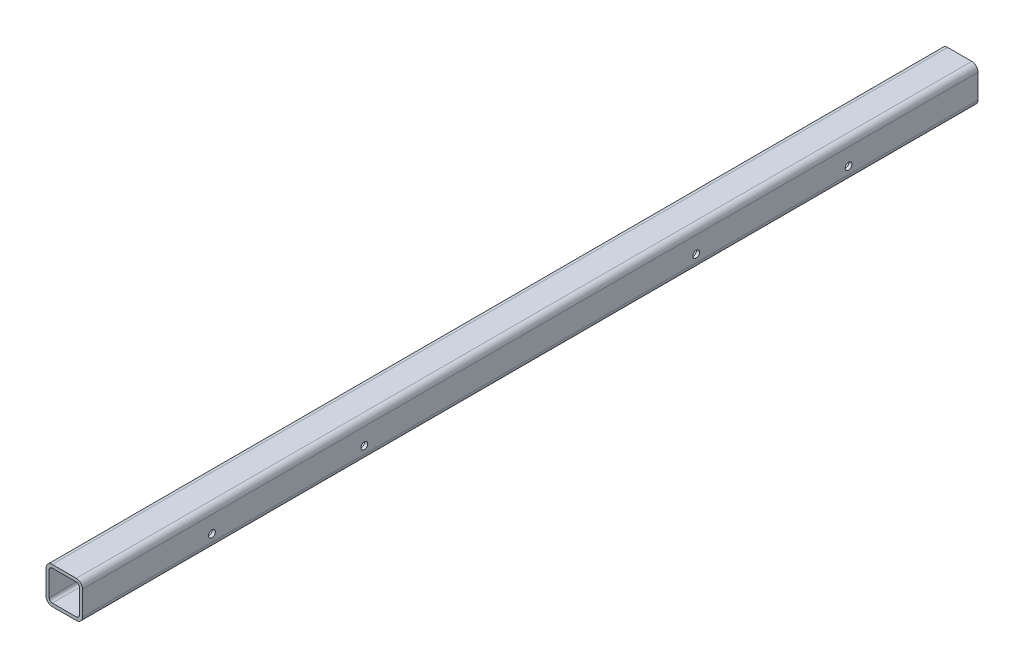
SolidWorks part; units mm, degrees
material "方管70×6/不锈钢304"
ref_plane "Front Plane" through (0, 0, 0) normal (0, 0, 1) x (1, 0, 0)
ref_plane "Top Plane" through (0, 0, 0) normal (0, 1, 0) x (1, 0, 0)
ref_plane "Right Plane" through (0, 0, 0) normal (1, 0, 0) x (0, 0, -1)
sketch "Sketch1" plane through (0, 0, 0) normal (0, 0, 1) x (1, 0, 0)
  line L1 (12, 0) -> (58, 0)
  line L2 (0, 12) -> (0, 58)
  line L3 (12, 70) -> (58, 70)
  line L4 (70, 12) -> (70, 58)
  line L5 (12, 6) -> (58, 6)
  line L6 (6, 12) -> (6, 58)
  line L7 (12, 64) -> (58, 64)
  line L8 (64, 12) -> (64, 58)
  arc A0 (12, 6) -> (6, 12) centre (12, 12) cw
  arc A1 (58, 6) -> (64, 12) centre (58, 12) ccw
  arc A2 (58, 64) -> (64, 58) centre (58, 58) cw
  arc A3 (6, 58) -> (12, 64) centre (12, 58) cw
  arc A4 (12, 0) -> (0, 12) centre (12, 12) cw
  arc A5 (58, 0) -> (70, 12) centre (58, 12) ccw
  arc A6 (58, 70) -> (70, 58) centre (58, 58) cw
  arc A7 (0, 58) -> (12, 70) centre (12, 58) cw
  point P19 (0, 0)
  point P22 (70, 0)
  point P27 (0, 70)
  dimension "D7" = 6
  dimension "D8" = 12
  dimension "D1" = 70
  dimension "D2" = 70
  dimension "D3" = 6
  dimension "D4" = 6
  dimension "D5" = 6
  dimension "D6" = 6
extrude "Boss-Extrude1" add sketch "Sketch1" along normal blind 1716
sketch "Sketch2" plane through (0, 0, 0) normal (-1, 0, 0) x (0, 0, 1)
  line L0 (0, 58) -> (0, 12) construction
  line L1 (1716, 0) -> (0, 0) construction
  circle A0 centre (248, 26) radius 6.5
  circle A1 centre (540, 26) radius 6.5
  dimension "D1" = 13
  dimension "D2" = 248
  dimension "D3" = 26
  dimension "D4" = 2
extrude "Cut-Extrude1" cut sketch "Sketch2" against normal through all
pattern_linear "LPattern1" count 2 spacing 928 along (0, 0, 1) of "Cut-Extrude1"
